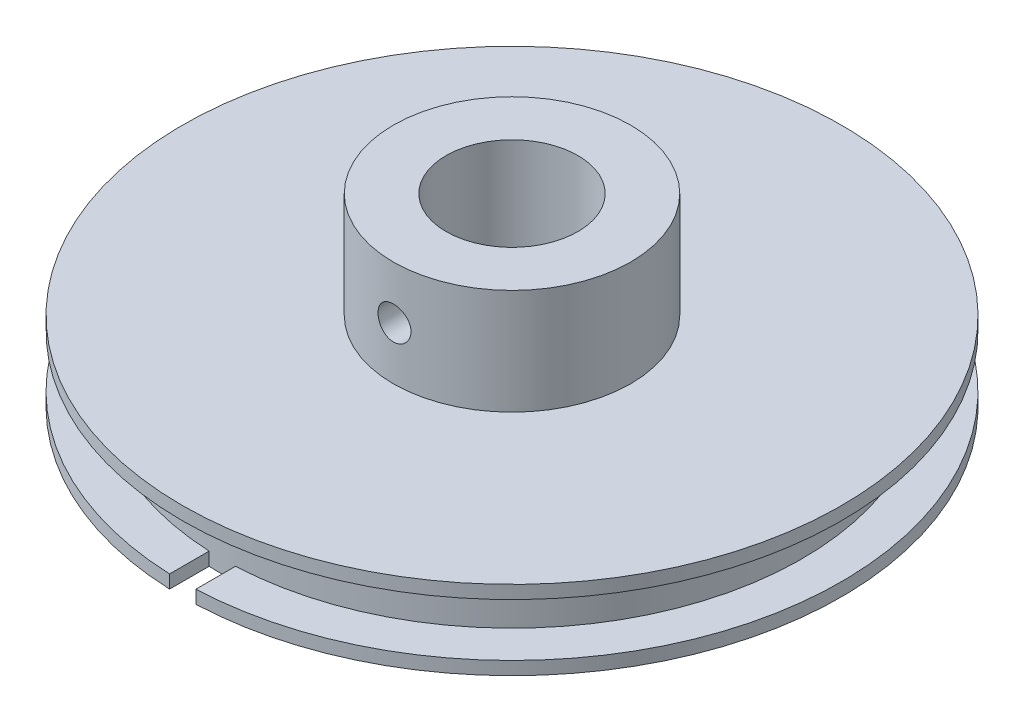
from build123d import *

# Parameters (mm, degrees)
CUT_EXTRUDE1_START    = -10
CUT_EXTRUDE1_DEPTH    = 10
M3_TAPPED_HOLE1_D     = 2.5
M3_TAPPED_HOLE1_DEPTH = 7.5
M3_TAPPED_HOLE1_TIP   = 0.751075774


with BuildPart() as part:
    # Sketch1 → Revolve1 (revolve)
    with BuildSketch(Plane.XY, mode=Mode.PRIVATE) as revolve1_sk:
        Polygon((-5, 0), (-9, 0), (-9, -8), (-25, -8), (-25, -9), (-22, -9), (-22, -13), (-25, -13), (-25, -14), (-5, -14), align=None)
    revolve(revolve1_sk.sketch.rotate(Axis((0, 0, 0), (0, -1, 0)), 270), axis=Axis((0, 0, 0), (0, -1, 0)))

    # Sketch2 → Cut-Extrude1 (cut)
    with BuildSketch(Plane(origin=(0, -13, 0), x_dir=(1, 0, 0), z_dir=(0, 1, 0)).offset(CUT_EXTRUDE1_START)):
        with BuildLine():
            Line((-1, -21.977260976), (-1, -40))
            Line((-1, -40), (1, -40))
            Line((1, -40), (1, -21.977260976))
            ThreePointArc((1, -21.977260976), (0, -22), (-1, -21.977260976))
        make_face()
    extrude(amount=CUT_EXTRUDE1_DEPTH, mode=Mode.SUBTRACT)

    # M3 Tapped Hole1
    with Locations(Plane(origin=(0, -4, 9), x_dir=(1, 0, 0), z_dir=(0, 0, 1))):
        with Locations((0, 0)):
            Hole(M3_TAPPED_HOLE1_D / 2, depth=M3_TAPPED_HOLE1_DEPTH)
            with Locations((0, 0, -(M3_TAPPED_HOLE1_DEPTH + M3_TAPPED_HOLE1_TIP / 2))):  # 118° drill point
                Cone(0, M3_TAPPED_HOLE1_D / 2, M3_TAPPED_HOLE1_TIP, mode=Mode.SUBTRACT)


solid = part.part
